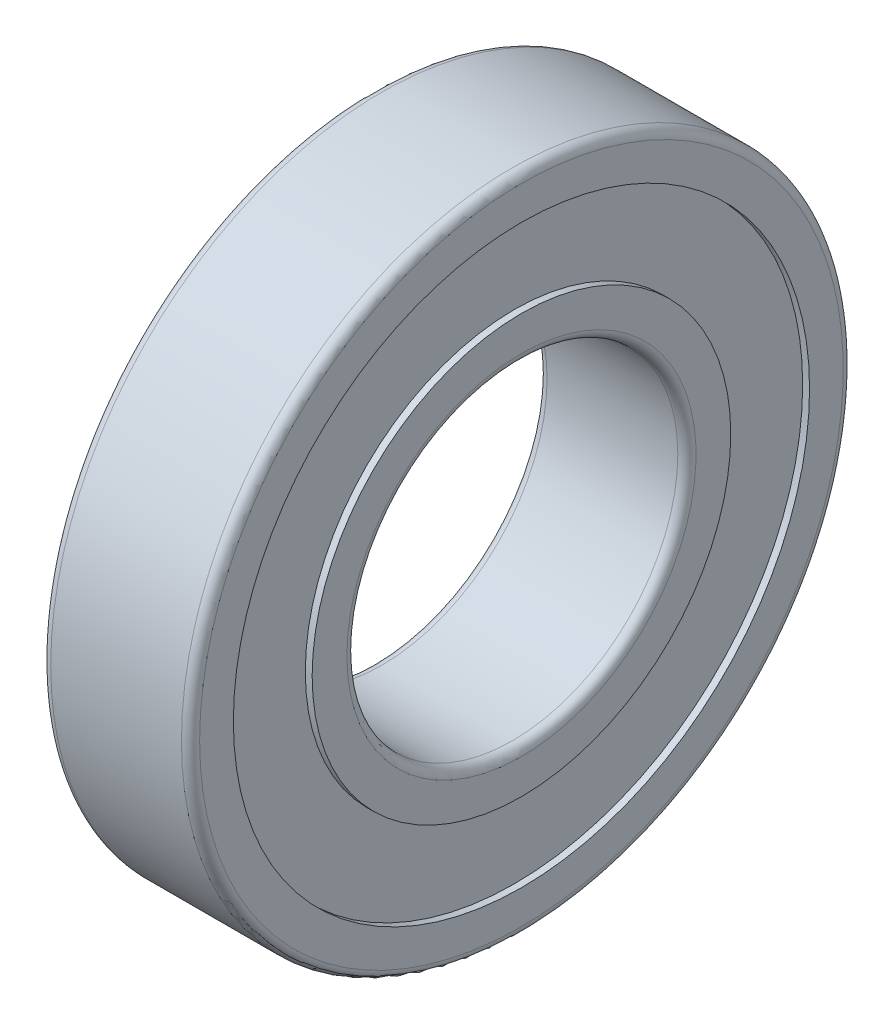
SolidWorks part; units mm, degrees
ref_plane "Front Plane" through (0, 0, 0) normal (0, 0, 1) x (1, 0, 0)
ref_plane "Top Plane" through (0, 0, 0) normal (0, 1, 0) x (1, 0, 0)
ref_plane "Right Plane" through (0, 0, 0) normal (1, 0, 0) x (0, 0, -1)
sketch "Sketch1" plane through (0, 0, 0) normal (0, 0, 1) x (1, 0, 0)
  line L0 (0, 0) -> (18, 0) construction
  line L1 (0, 20) -> (18, 20)
  line L2 (0, 40) -> (18, 40)
  line L3 (0, 40) -> (0, 34.825)
  line L4 (0, 34.825) -> (0.83, 34.825)
  line L5 (18, 40) -> (18, 34.825)
  line L6 (0.83, 34.825) -> (0.83, 25.3)
  line L7 (0.83, 25.3) -> (0, 25.3)
  line L8 (0, 25.3) -> (0, 20)
  line L9 (18, 34.825) -> (17.17, 34.825)
  line L10 (17.17, 34.825) -> (17.17, 25.3)
  line L11 (17.17, 25.3) -> (18, 25.3)
  line L12 (18, 25.3) -> (18, 20)
  dimension "D" = 80
  dimension "B" = 18
  dimension "D_s" = 40
  dimension "MSM_1" = 69.65
  dimension "MSM_2" = 50.6
  dimension "MSM_3" = 0.83
revolve "Revolve1" add sketch "Sketch1" angle 360 about L0
fillet "Fillet1" radius 1.1 2 edges at (18, 0, 40) (0, 0, 40)
fillet "Fillet2" radius 1.1 2 edges at (18, 0, 20) (0, 0, 20)
